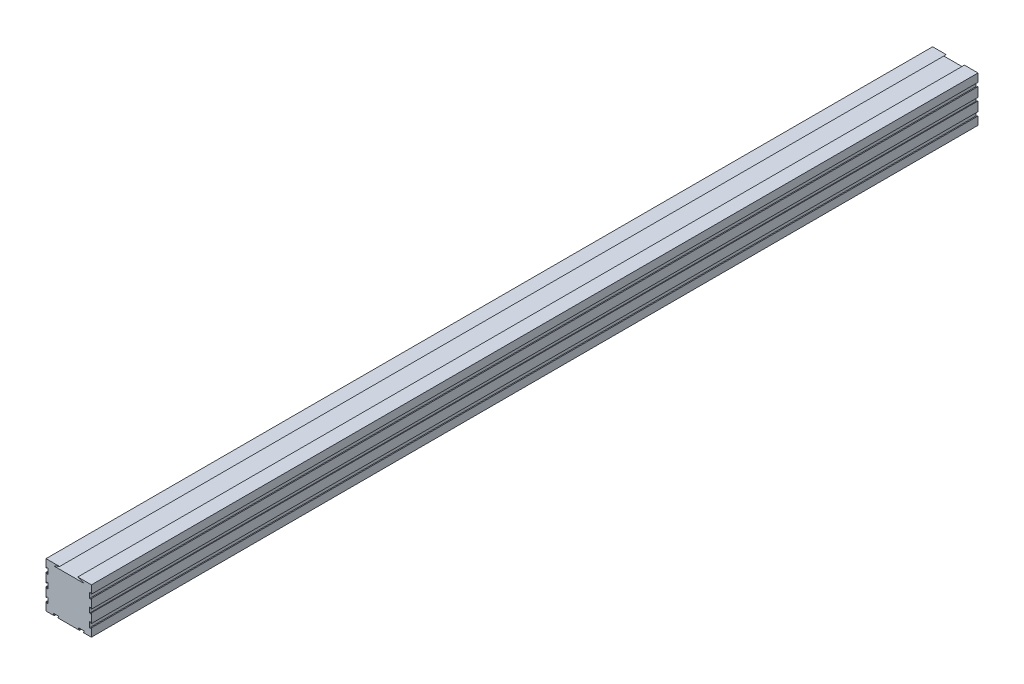
from build123d import *

# Parameters (mm, degrees)
SKETCH_1_W               = 75
SKETCH_1_H               = 75
EXTRUDE_1_DEPTH          = 732.5
CUT_EXTRUDE_1_DEPTH      = 732.5
CUT_EXTRUDE_2_DEPTH      = 1465
CUT_EXTRUDE_3_DEPTH      = 1466.959583345
CUT_EXTRUDE_3_DEPTH_BACK = 1466.959583345


with BuildPart() as part:
    # 草图1 → 凸台-拉伸1 (new, symmetric)
    with BuildSketch(Plane.XY):
        Rectangle(SKETCH_1_W, SKETCH_1_H)
    extrude(amount=EXTRUDE_1_DEPTH, both=True)

    # 草图2 → 切除-拉伸1 (cut, symmetric)
    with BuildSketch(Plane.XY):
        Polygon((-17.9, -36.8), (-16.55, -36.8), (-16.55, -34.5), (-25.45, -34.5), (-25.45, -36.8), (-24.1, -36.8), (-24.1, -37.5), (-17.9, -37.5), align=None)
        Polygon((16.55, -34.5), (16.55, -36.8), (17.9, -36.8), (17.9, -37.5), (24.1, -37.5), (24.1, -36.8), (25.45, -36.8), (25.45, -34.5), align=None)
    extrude(amount=CUT_EXTRUDE_1_DEPTH, both=True, mode=Mode.SUBTRACT)

    # 草图3 → 切除-拉伸2 (cut)
    with BuildSketch(Plane.XY.offset(732.5)):
        Polygon((37.5, 2.6), (36.8, 2.6), (36.8, 4.45), (34.5, 4.45), (34.5, -4.45), (36.8, -4.45), (36.8, -2.6), (37.5, -2.6), align=None)
        Polygon((37.5, -17.9), (36.8, -17.9), (36.8, -16.55), (34.5, -16.55), (34.5, -25.45), (36.8, -25.45), (36.8, -24.1), (37.5, -24.1), align=None)
        Polygon((36.8, 24.1), (36.8, 25.45), (34.5, 25.45), (34.5, 16.55), (36.8, 16.55), (36.8, 17.9), (37.5, 17.9), (37.5, 24.1), align=None)
    cut_extrude_2 = extrude(amount=-CUT_EXTRUDE_2_DEPTH, mode=Mode.SUBTRACT)

    # 镜向1: 切除-拉伸2 across plane
    add(cut_extrude_2.mirror(Plane(origin=(0, 0, 0), x_dir=(0, 0, 1), z_dir=(1, 0, 0))), mode=Mode.SUBTRACT)

    # 草图4 → 切除-拉伸3 (cut, two sides: drawn at the far end of the back side and taken through both)
    with BuildSketch(Plane.XY.offset(732.5).offset(-CUT_EXTRUDE_3_DEPTH_BACK)):
        Polygon((164.287302387, 109.214920955), (-15, 37.5), (-25, 33.5), (25, 33.5), (15, 37.5), (-164.287302387, 109.214920955), (-164.287302387, -276.981747517), (164.287302387, -276.981747517), align=None)
    extrude(amount=CUT_EXTRUDE_3_DEPTH + CUT_EXTRUDE_3_DEPTH_BACK, mode=Mode.SUBTRACT)


solid = part.part
